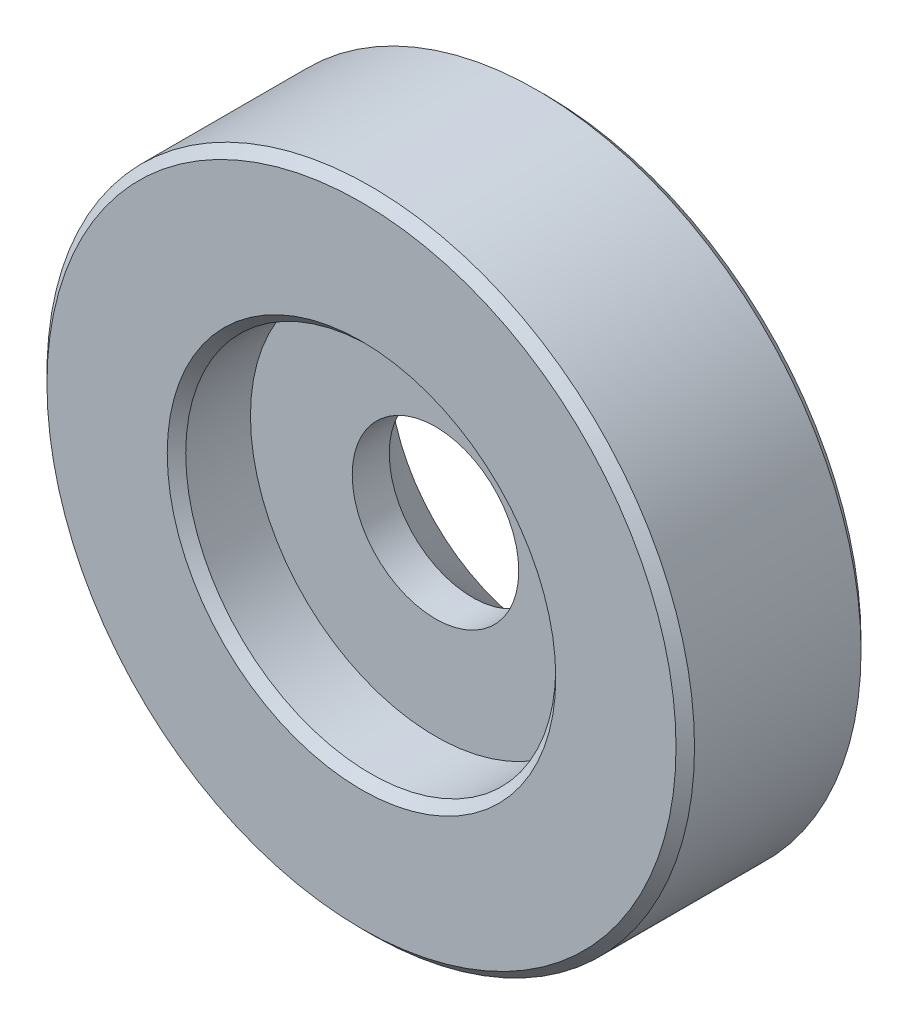
from build123d import *

# Parameters (mm, degrees)
SKETCH1_R                                           = 17.5
BOSS_EXTRUDE1_DEPTH                                 = 10
CHAMFER1_SIZE                                       = 0.5
HOLE_SIZE_PER_SOCKET_FLAT_COUNTEBLZKK_H_D           = 9
HOLE_SIZE_PER_SOCKET_FLAT_COUNTEBLZKK_H_CSINK_D     = 17
HOLE_SIZE_PER_SOCKET_FLAT_COUNTEBLZKK_H_CSINK_ANGLE = 90
SKETCH5_R                                           = 10
CUT_EXTRUDE1_DEPTH                                  = 4
CHAMFER2_SIZE                                       = 0.5


with BuildPart() as part:
    # Sketch1 → Boss-Extrude1 (new body)
    with BuildSketch(Plane.XY):
        Circle(SKETCH1_R)
    extrude(amount=BOSS_EXTRUDE1_DEPTH)

    # Chamfer1
    chamfer1_edges = [part.edges().sort_by_distance(p)[0] for p in [
        (-17.5, 0, 0),
        (-17.5, 0, 10),
    ]]
    chamfer(chamfer1_edges, length=CHAMFER1_SIZE)

    # Hole size (per socket flat counteBLZKk head screw type)1 (through all)
    with Locations(Plane(origin=(0, 0, 0), x_dir=(1, 0, 0), z_dir=(0, 0, -1))):
        with Locations((0, 0)):
            CounterSinkHole(HOLE_SIZE_PER_SOCKET_FLAT_COUNTEBLZKK_H_D / 2, HOLE_SIZE_PER_SOCKET_FLAT_COUNTEBLZKK_H_CSINK_D / 2, counter_sink_angle=HOLE_SIZE_PER_SOCKET_FLAT_COUNTEBLZKK_H_CSINK_ANGLE)

    # Sketch5 → Cut-Extrude1 (cut)
    with BuildSketch(Plane.XY.offset(10)):
        Circle(SKETCH5_R)
    extrude(amount=-CUT_EXTRUDE1_DEPTH, mode=Mode.SUBTRACT)

    # Chamfer2
    chamfer2_edges = [part.edges().sort_by_distance(p)[0] for p in [
        (-10, 0, 10),
    ]]
    chamfer(chamfer2_edges, length=CHAMFER2_SIZE)


solid = part.part
